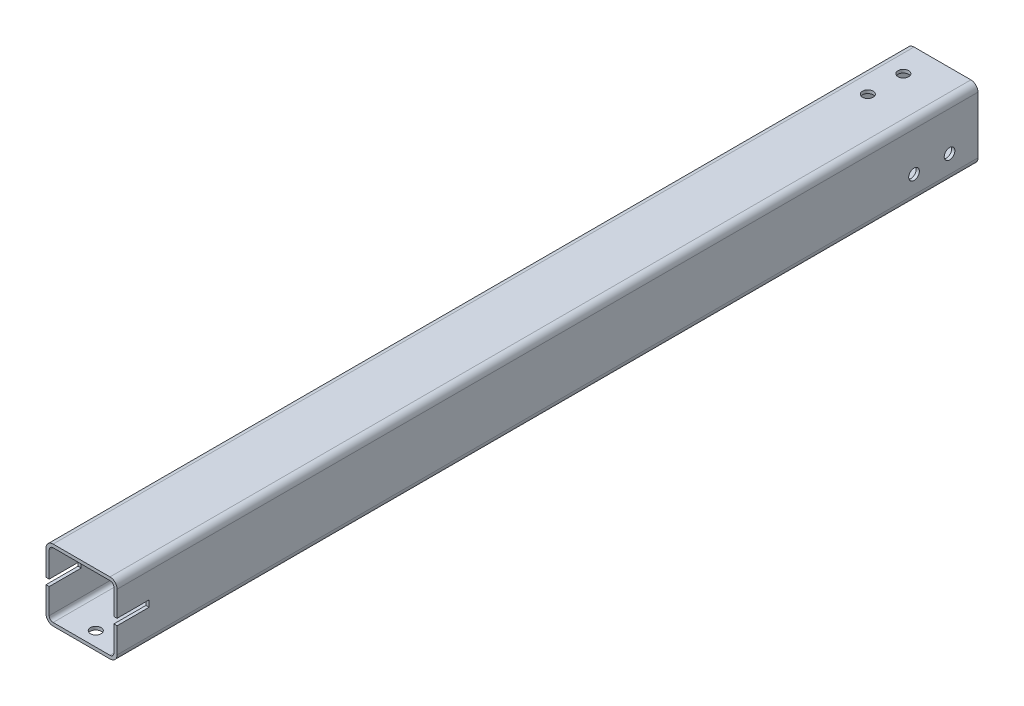
from build123d import *

# Parameters (mm, degrees)
BOSS_EXTRUDE1_DEPTH = 1211
CUT_EXTRUDE1_REACH  = 1218.15
SKETCH_1_R          = 7.5
CUT_EXTRUDE2_REACH  = 1218.15
SKETCH2_R           = 7.5
CUT_EXTRUDE3_REACH  = 1218.15
SKETCH3_R           = 7.5
SKETCH4_W           = 45
SKETCH4_H           = 9
CUT_EXTRUDE4_DEPTH  = 1217.150072976


with BuildPart() as part:
    # Sketch1 → Boss-Extrude1 (new body)
    with BuildSketch(Plane.XY):
        with BuildLine():
            Line((-40, -50), (40, -50))
            ThreePointArc((40, -50), (47.071067812, -47.071067812), (50, -40))
            Line((50, -40), (50, 40))
            ThreePointArc((50, 40), (47.071067812, 47.071067812), (40, 50))
            Line((40, 50), (-40, 50))
            ThreePointArc((-40, 50), (-47.071067812, 47.071067812), (-50, 40))
            Line((-50, 40), (-50, -40))
            ThreePointArc((-50, -40), (-47.071067812, -47.071067812), (-40, -50))
        make_face()
        with BuildLine():
            Line((-40, -45.5), (40, -45.5))
            ThreePointArc((40, -45.5), (43.889087297, -43.889087297), (45.5, -40))
            Line((45.5, -40), (45.5, 40))
            ThreePointArc((45.5, 40), (43.889087297, 43.889087297), (40, 45.5))
            Line((40, 45.5), (-40, 45.5))
            ThreePointArc((-40, 45.5), (-43.889087297, 43.889087297), (-45.5, 40))
            Line((-45.5, 40), (-45.5, -40))
            ThreePointArc((-45.5, -40), (-43.889087297, -43.889087297), (-40, -45.5))
        make_face(mode=Mode.SUBTRACT)
    extrude(amount=BOSS_EXTRUDE1_DEPTH)

    # 草图1 → Cut-Extrude1 (cut, up to next)
    with BuildSketch(Plane(origin=(50, 0, 0), x_dir=(0, 0, -1), z_dir=(1, 0, 0)), mode=Mode.PRIVATE) as cut_extrude1_sk1:
        with Locations((-40, -15)):
            Circle(SKETCH_1_R)
    cut_extrude1_tool1 = extrude(cut_extrude1_sk1.sketch, amount=-CUT_EXTRUDE1_REACH, mode=Mode.PRIVATE) & part.part
    # 草图1 → Cut-Extrude1 (cut, up to next)
    with BuildSketch(Plane(origin=(50, 0, 0), x_dir=(0, 0, -1), z_dir=(1, 0, 0)), mode=Mode.PRIVATE) as cut_extrude1_sk2:
        with Locations((-90, -15)):
            Circle(SKETCH_1_R)
    cut_extrude1_tool2 = extrude(cut_extrude1_sk2.sketch, amount=-CUT_EXTRUDE1_REACH, mode=Mode.PRIVATE) & part.part
    add(cut_extrude1_tool1.solids().sort_by_distance((50, -15, 40))[0], mode=Mode.SUBTRACT)
    add(cut_extrude1_tool2.solids().sort_by_distance((50, -15, 90))[0], mode=Mode.SUBTRACT)

    # Sketch2 → Cut-Extrude2 (cut, up to next)
    with BuildSketch(Plane.XZ.offset(50), mode=Mode.PRIVATE) as cut_extrude2_sk1:
        with Locations(Location((0, 20, 0), (0, 0, 270))):
            Circle(SKETCH2_R)
    cut_extrude2_tool1 = extrude(cut_extrude2_sk1.sketch, amount=-CUT_EXTRUDE2_REACH, mode=Mode.PRIVATE) & part.part
    # Sketch2 → Cut-Extrude2 (cut, up to next)
    with BuildSketch(Plane.XZ.offset(50), mode=Mode.PRIVATE) as cut_extrude2_sk2:
        with Locations(Location((0, 90, 0), (0, 0, 270))):
            Circle(SKETCH2_R)
    cut_extrude2_tool2 = extrude(cut_extrude2_sk2.sketch, amount=-CUT_EXTRUDE2_REACH, mode=Mode.PRIVATE) & part.part
    # Sketch2 → Cut-Extrude2 (cut, up to next)
    with BuildSketch(Plane.XZ.offset(50), mode=Mode.PRIVATE) as cut_extrude2_sk3:
        with Locations(Location((0, 1191, 0), (0, 0, 270))):
            Circle(SKETCH2_R)
    cut_extrude2_tool3 = extrude(cut_extrude2_sk3.sketch, amount=-CUT_EXTRUDE2_REACH, mode=Mode.PRIVATE) & part.part
    add(cut_extrude2_tool1.solids().sort_by_distance((0, -50, 20))[0], mode=Mode.SUBTRACT)
    add(cut_extrude2_tool2.solids().sort_by_distance((0, -50, 90))[0], mode=Mode.SUBTRACT)
    add(cut_extrude2_tool3.solids().sort_by_distance((0, -50, 1191))[0], mode=Mode.SUBTRACT)

    # Sketch3 → Cut-Extrude3 (cut, up to next)
    with BuildSketch(Plane(origin=(0, 50, 0), x_dir=(1, 0, 0), z_dir=(0, 1, 0)), mode=Mode.PRIVATE) as cut_extrude3_sk1:
        with Locations(Location((-15, -40, 0), (0, 0, 270))):
            Circle(SKETCH3_R)
    cut_extrude3_tool1 = extrude(cut_extrude3_sk1.sketch, amount=-CUT_EXTRUDE3_REACH, mode=Mode.PRIVATE) & part.part
    # Sketch3 → Cut-Extrude3 (cut, up to next)
    with BuildSketch(Plane(origin=(0, 50, 0), x_dir=(1, 0, 0), z_dir=(0, 1, 0)), mode=Mode.PRIVATE) as cut_extrude3_sk2:
        with Locations(Location((-15, -90, 0), (0, 0, 270))):
            Circle(SKETCH3_R)
    cut_extrude3_tool2 = extrude(cut_extrude3_sk2.sketch, amount=-CUT_EXTRUDE3_REACH, mode=Mode.PRIVATE) & part.part
    add(cut_extrude3_tool1.solids().sort_by_distance((-15, 50, 40))[0], mode=Mode.SUBTRACT)
    add(cut_extrude3_tool2.solids().sort_by_distance((-15, 50, 90))[0], mode=Mode.SUBTRACT)

    # Sketch4 → Cut-Extrude4 (cut, through all)
    with BuildSketch(Plane(origin=(50, 0, 0), x_dir=(0, 0, -1), z_dir=(1, 0, 0))):
        with Locations((-1188.5, 0)):
            Rectangle(SKETCH4_W, SKETCH4_H)
    extrude(amount=-CUT_EXTRUDE4_DEPTH, mode=Mode.SUBTRACT)


solid = part.part
